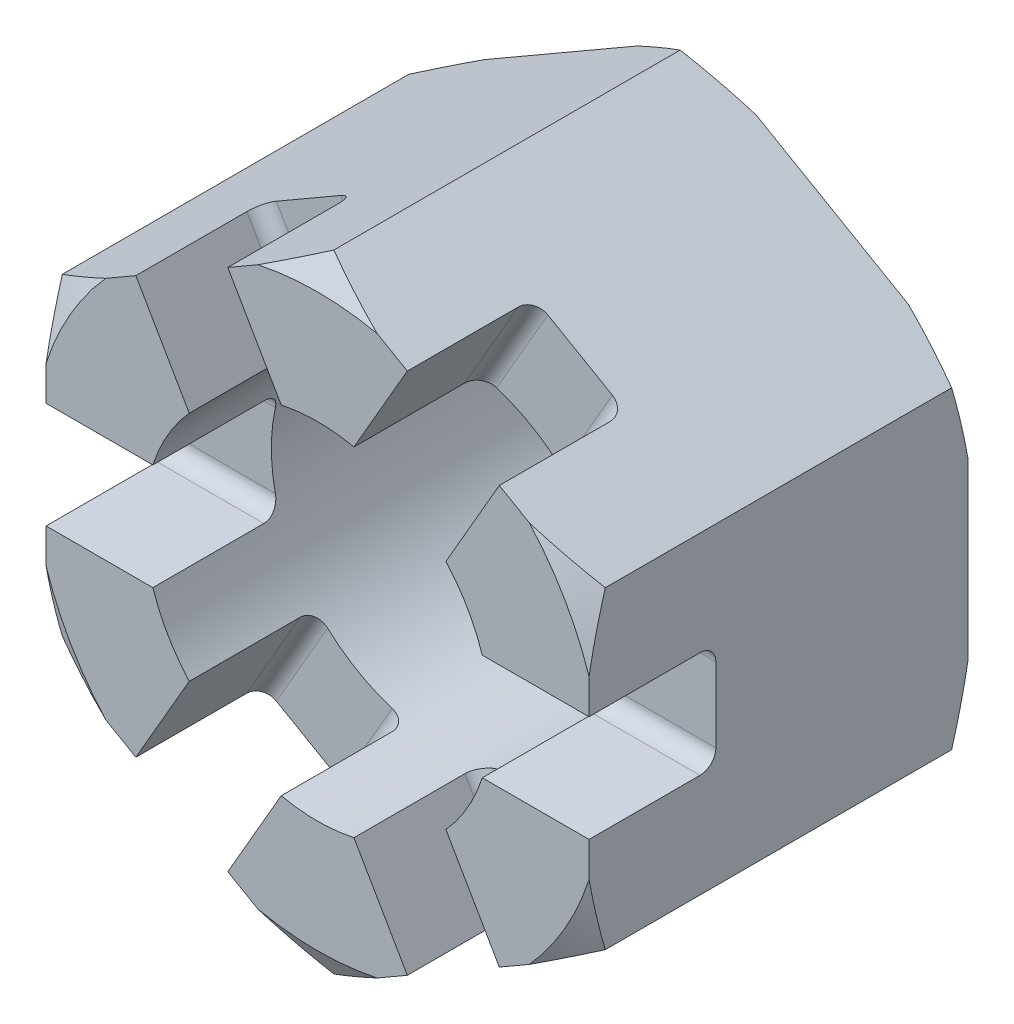
SolidWorks part; units mm, degrees
ref_plane "基准面1" through (0, 0, 0) normal (0, 0, 1) x (1, 0, 0)
ref_plane "基准面2" through (0, 0, 0) normal (0, 1, 0) x (1, 0, 0)
ref_plane "基准面3" through (0, 0, 0) normal (1, 0, 0) x (0, 0, -1)
sketch "尺寸草图" plane through (0, 0, 0) normal (0, 0, 1) x (1, 0, 0)
  line L0 (0, 0) -> (36, 0) construction
  line L1 (39.55, 0) -> (65.45, 0) construction
  line L2 (65.45, 0) -> (98.65, 0) construction
  line L3 (-20.8571, 0) -> (2, 0) construction
  line L4 (0, 0) -> (39.55, 0) construction
  point P3 (24, 0)
  point P4 (2, 0)
  point P5 (39.55, 0)
  point P6 (23.9, 0)
  point P8 (36, 0)
  point P15 (55.45, 0)
  point P16 (72.15, 0)
  dimension "D1" = 22.8571
  dimension "D" = 24
  dimension "P" = 2
  dimension "e(最小)" = 39.55
  dimension "m(最大)" = 23.9
  dimension "s(最大)" = 36
  dimension "da" = 25.9
  dimension "dw" = 33.2
  dimension "w(最大)" = 15.9
  dimension "n(最大)" = 6.7
sketch "草图1" plane through (0, 0, 0) normal (0, 0, 1) x (1, 0, 0)
  line L0 (-17.1257, 0) -> (17.1257, 0) construction
  line L1 (0, 19.775) -> (0, -19.775) construction
  line L3 (0, 19.775) -> (-17.1257, 9.8875)
  line L4 (-17.1257, 9.8875) -> (-17.1257, -9.8875)
  line L5 (-17.1257, -9.8875) -> (0, -19.775)
  line L6 (0, -19.775) -> (17.1257, -9.8875)
  line L7 (17.1257, -9.8875) -> (17.1257, 9.8875)
  line L8 (17.1257, 9.8875) -> (0, 19.775)
  circle A0 centre (0, 0) radius 17.1257 construction
  circle A1 centre (0, 0) radius 10.9175
  dimension "D" = 21.835
  dimension "e" = 39.55
extrude "基体-拉伸" add sketch "草图1" along normal blind 23.9
cosmetic thread "装饰螺纹线1" parameters "D2"=24
sketch "草图2" plane through (0, 0, 0) normal (0, 0, -1) x (-1, 0, 0)
  circle A0 centre (0, 0) radius 18
  circle A1 centre (0, 0) radius 10.9175 construction
  dimension "s" = 36
extrude "切除-拉伸1" cut sketch "草图2" against normal through all draft 60 flip side to cut
sketch "草图3" plane through (0, 0, 23.9) normal (0, 0, 1) x (1, 0, 0)
  circle A0 centre (0, 0) radius 18
  dimension "D1" = 36
extrude "切除-拉伸2" cut sketch "草图3" against normal through all draft 60 flip side to cut
sketch "草图6" plane through (17.1257, 0, 0) normal (1, 0, 0) x (0, 0, -1)
  line L0 (-14.9451, 0) -> (3.4921, 0) construction
  line L1 (-23.9, 0) -> (0, 0) construction
  line L3 (-23.9, -5.5418) -> (-23.9, 5.5418) construction
  line L4 (-23.9, -3.35) -> (-23.9, 3.35)
  line L5 (-23.9, 3.35) -> (-16.9, 3.35)
  line L6 (-15.9, -2.35) -> (-15.9, 2.35)
  line L7 (0, -5.5418) -> (0, 5.5418) construction
  line L8 (-23.9, -3.35) -> (-16.9, -3.35)
  arc A0 (-16.9, 3.35) -> (-15.9, 2.35) centre (-16.9, 2.35) cw
  arc A1 (-16.9, -3.35) -> (-15.9, -2.35) centre (-16.9, -2.35) ccw
  point P14 (-15.9, 3.35)
  point P17 (-15.9, -3.35)
  dimension "D1" = 1
  dimension "W" = 15.9
  dimension "n" = 3.35
extrude "切除-拉伸3" cut sketch "草图6" against normal through all
pattern_circular "阵列(圆周)1" count 3 over 360 about axis through (0, 0, 0) along (0, 0, 1) of "切除-拉伸3"
chamfer "倒角1" distance 0.3804 angle 45 1 edges at (10.9175, 0, 0)
